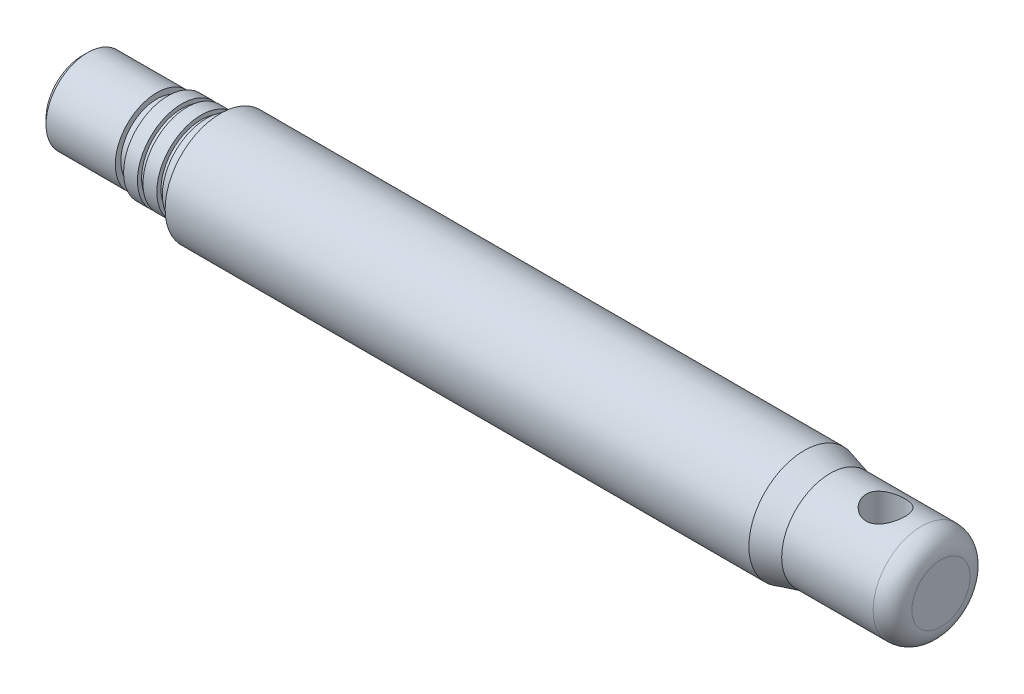
from build123d import *

# Parameters (mm, degrees)
CUT_EXTRUDE_1_DEPTH      = 312.287648325
CUT_EXTRUDE_1_DEPTH_BACK = 312.287648325
SKETCH_2_R               = 7
CHAMFER_1_SIZE           = 2
FILLET_1_R               = 7


with BuildPart() as part:
    # 草图1 → 旋转1 (revolve)
    with BuildSketch(Plane.XY, mode=Mode.PRIVATE) as revolve_1_sk:
        Polygon((0, 0), (0, 15), (27, 15), (27, 13), (31, 13), (31, 16), (36, 16), (36, 14.5), (38, 14.5), (38, 16), (43, 16), (43, 14.5), (45, 14.5), (45, 16), (50, 16), (50, 20), (260.669872981, 20), (270, 17.5), (310, 17.5), (310, 0), align=None)
    revolve(revolve_1_sk.sketch.rotate(Axis((0, 0, 0), (1, 0, 0)), 90), axis=Axis((0, 0, 0), (1, 0, 0)))

    # 草图2 → 切除-拉伸1 (cut, two sides: drawn at the far end of the back side and taken through both)
    with BuildSketch(Plane(origin=(0, 0, 0), x_dir=(1, 0, 0), z_dir=(0, 1, 0)).offset(-CUT_EXTRUDE_1_DEPTH_BACK)):
        with Locations(Location((290, 0, 0), (0, 0, 270))):
            Circle(SKETCH_2_R)
    extrude(amount=CUT_EXTRUDE_1_DEPTH + CUT_EXTRUDE_1_DEPTH_BACK, mode=Mode.SUBTRACT)

    # 倒角1
    chamfer_1_edges = [part.edges().sort_by_distance(p)[0] for p in [
        (0, 0, -15),
    ]]
    chamfer(chamfer_1_edges, length=CHAMFER_1_SIZE)

    # 圆角1
    fillet_1_edges = [part.edges().sort_by_distance(p)[0] for p in [
        (310, 0, -17.5),
    ]]
    fillet(fillet_1_edges, radius=FILLET_1_R)


solid = part.part
